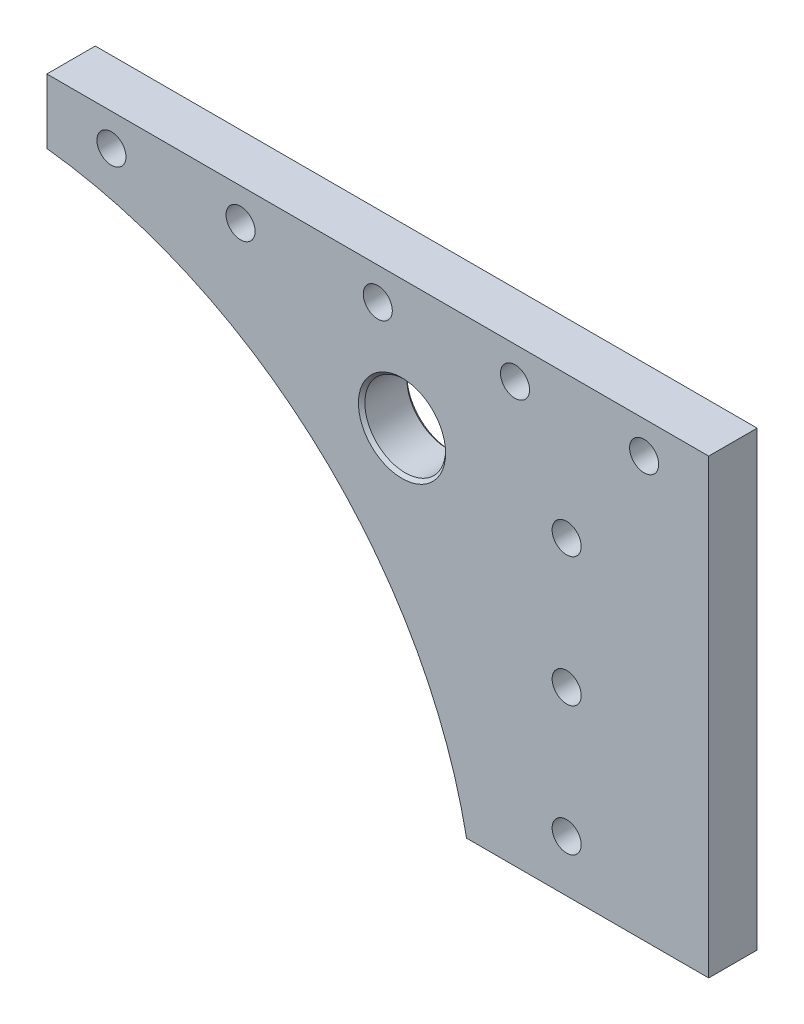
from build123d import *

# Parameters (mm, degrees)
EXTRUDE_1_DEPTH              = 7.5
HOLE_WIZARD_M8_2_D           = 9
HOLE_WIZARD_M8_2_CBORE_D     = 15
HOLE_WIZARD_M8_2_CBORE_DEPTH = 8.6
HOLE_WIZARD_M5_1_D           = 4.2
HOLE_WIZARD_M5_1_DEPTH       = 12.4
HOLE_WIZARD_M5_1_TIP         = 1.2618073
SKETCH_11_R                  = 150
CUT_EXTRUDE_4_DEPTH          = 249.696602309
SKETCH_12_R                  = 12.5
CUT_EXTRUDE_5_DEPTH          = 249.696602309
CHAMFER_1_SIZE               = 1


with BuildPart() as part:
    # 草图1 → 凸台-拉伸1 (new, symmetric)
    with BuildSketch(Plane.XY):
        Polygon((0, 0), (205, 0), (205, -140), (130, -140), (0, -20), align=None)
    extrude(amount=EXTRUDE_1_DEPTH, both=True)

    # M8 六角凹头螺钉的柱形沉头孔2 (through all)
    with Locations(Plane(origin=(0, 0, -7.5), x_dir=(1, 0, 0), z_dir=(0, 0, -1))):
        with Locations((20, 10), (60, 10), (102.5, 10), (145, 10), (161, 44), (161, 84), (161, 124), (185, 10)):
            CounterBoreHole(HOLE_WIZARD_M8_2_D / 2, HOLE_WIZARD_M8_2_CBORE_D / 2, HOLE_WIZARD_M8_2_CBORE_DEPTH)

    # M5 螺纹孔1
    with Locations(Plane(origin=(0, 0, -7.5), x_dir=(1, 0, 0), z_dir=(0, 0, -1))):
        with Locations((40, 10), (123.75, 10), (161, 64), (161, 104)):
            Hole(HOLE_WIZARD_M5_1_D / 2, depth=HOLE_WIZARD_M5_1_DEPTH)
            with Locations((0, 0, -(HOLE_WIZARD_M5_1_DEPTH + HOLE_WIZARD_M5_1_TIP / 2))):  # 118° drill point
                Cone(0, HOLE_WIZARD_M5_1_D / 2, HOLE_WIZARD_M5_1_TIP, mode=Mode.SUBTRACT)

    # 草图11 → 切除-拉伸4 (cut, through all)
    with BuildSketch(Plane.XY.offset(7.5)):
        with Locations((-17.167132722, -169.014393782)):
            Circle(SKETCH_11_R)
    extrude(amount=-CUT_EXTRUDE_4_DEPTH, mode=Mode.SUBTRACT)

    # 草图12 → 切除-拉伸5 (cut, through all)
    with BuildSketch(Plane(origin=(0, 0, -7.5), x_dir=(-1, 0, 0), z_dir=(0, 0, -1))):
        with Locations((-110, -40)):
            Circle(SKETCH_12_R)
    extrude(amount=-CUT_EXTRUDE_5_DEPTH, mode=Mode.SUBTRACT)

    # 倒角1
    chamfer_1_edges = [part.edges().sort_by_distance(p)[0] for p in [
        (122.5, -40, 7.5),
        (122.5, -40, -7.5),
    ]]
    chamfer(chamfer_1_edges, length=CHAMFER_1_SIZE)


solid = part.part
